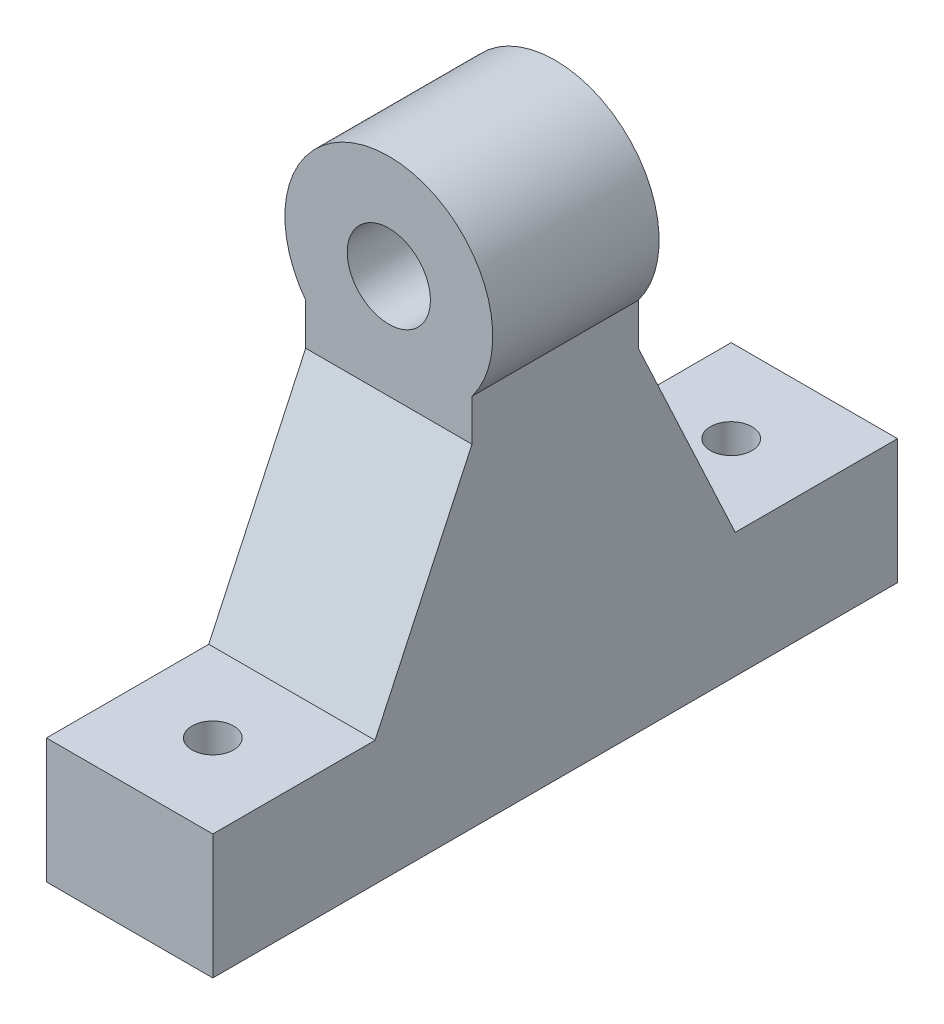
SolidWorks part; units mm, degrees
material "1060 合金"
ref_plane "前视基准面" through (0, 0, 0) normal (0, 0, 1) x (1, 0, 0)
ref_plane "上视基准面" through (0, 0, 0) normal (0, 1, 0) x (1, 0, 0)
ref_plane "右视基准面" through (0, 0, 0) normal (1, 0, 0) x (0, 0, -1)
sketch "草图1" plane through (0, 0, 0) normal (0, 0, 1) x (1, 0, 0)
  circle A0 centre (0, 0) radius 12.5
  circle A1 centre (0, 0) radius 5
  dimension "D1" = 10
  dimension "D2" = 25
extrude "凸台-拉伸1" add sketch "草图1" along normal mid plane 20
sketch "草图5" plane through (0, 0, 0) normal (1, 0, 0) x (0, 0, -1)
  line L0 (10, -12.5) -> (21.6577, -37.5)
  line L1 (21.6577, -37.5) -> (41.1684, -37.5)
  line L2 (41.1684, -37.5) -> (41.1684, -52.5)
  line L3 (41.1684, -52.5) -> (-41.1684, -52.5)
  line L6 (-10, -12.5) -> (10, -12.5)
  line L7 (-41.1684, -37.5) -> (-41.1684, -52.5)
  line L8 (-21.6577, -37.5) -> (-41.1684, -37.5)
  line L9 (-10, -12.5) -> (-21.6577, -37.5)
  dimension "D1" = 40
  dimension "D2" = 15
  dimension "D3" = 15
extrude "凸台-拉伸3" add sketch "草图5" along normal mid plane 20 separate body
sketch "草图6" plane through (0, -12.5, 0) normal (0, 1, 0) x (1, 0, 0)
  line L4 (-10, 10) -> (-10, -10)
  line L5 (-10, -10) -> (10, -10)
  line L6 (10, -10) -> (10, 10)
  line L7 (10, 10) -> (-10, 10)
  line L8 (-10, 10) -> (-10, -10)
  line L9 (-10, -10) -> (10, -10)
  line L10 (10, -10) -> (10, 10)
  line L11 (10, 10) -> (-10, 10)
  dimension "D1" = 0
extrude "凸台-拉伸4" add sketch "草图6" along normal up to surface up to face at (12.5, 0, 10)
hole_wizard "M6 螺纹孔1" positions "3D草图1" profile "草图8" tap size "M6" standard "GB" end condition up to next
sketch3d "3D草图1"
  line L0 (10, -37.5, -41.1684) -> (10, -37.5, -21.6577) construction
  line L1 (10, -37.5, -41.1684) -> (-10, -37.5, -41.1684) construction
  point P0 (0, -37.5, -31.1684)
  dimension "D1" = 10
  dimension "D2" = 10
sketch "草图8" plane through (0, -37.5, -31.1684) normal (1, 0, 0) x (0, 0, 1)
  line L0 (0, 0) -> (0, 15)
  line L1 (0, 15) -> (2.5, 15)
  line L2 (2.5, 15) -> (2.5, 0)
  line L5 (2.5, 0) -> (0, 0)
  line L11 (0, -6.35) -> (0, 107.95) construction
  dimension "通孔螺纹孔钻头直径" = 5
  dimension "通孔螺纹孔钻头深度" = 15
cosmetic thread "孔螺蚊线1" parameters "D2"=6
mirror "镜向1" about plane through (0, 0, 0) normal (0, 0, 1) of "M6 螺纹孔1"
